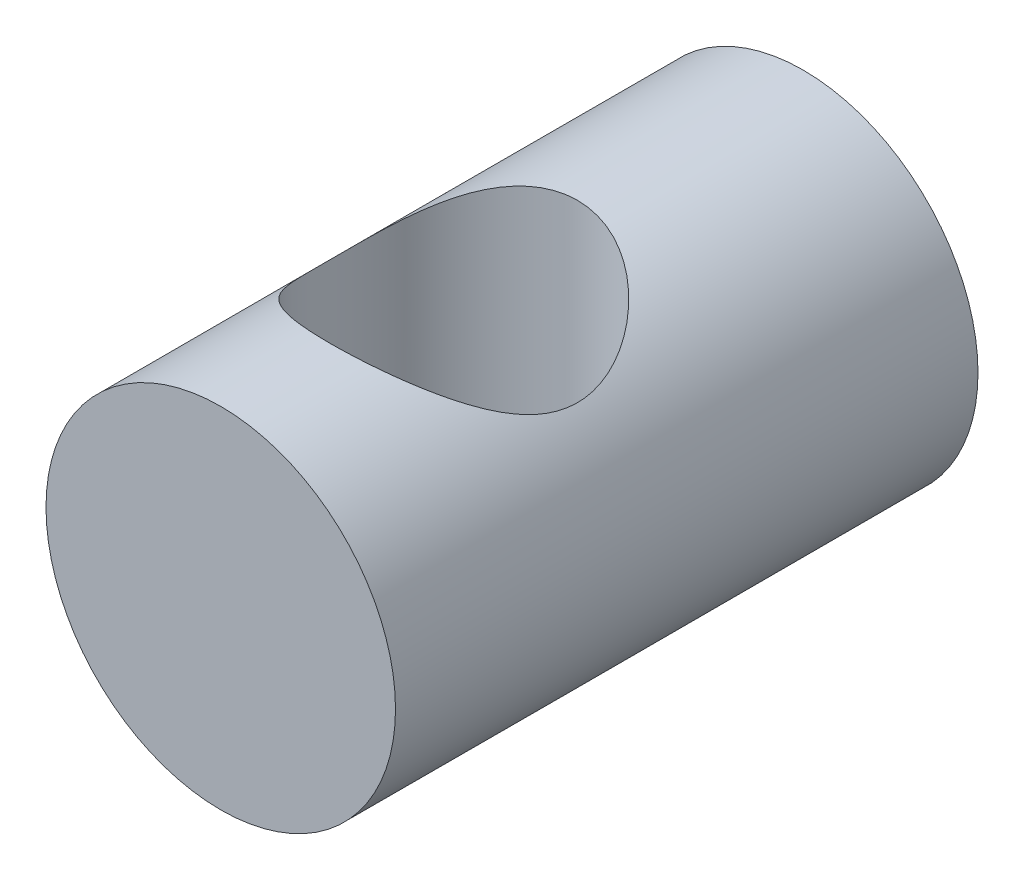
from build123d import *

# Parameters (mm, degrees)
SKETCH1_R              = 6
BOSS_EXTRUDE1_DEPTH    = 20
SKETCH5_W              = 4.25
SKETCH5_H              = 6
M10_TAPPED_HOLE1_D     = 8.5
M10_TAPPED_HOLE1_DEPTH = 27.5
M10_TAPPED_HOLE1_TIP   = 2.553657631


with BuildPart() as part:
    # Sketch1 → Boss-Extrude1 (new body)
    with BuildSketch(Plane.XY):
        Circle(SKETCH1_R)
    extrude(amount=BOSS_EXTRUDE1_DEPTH)

    # Sketch5 → M10 Tapped Hole2 (revolve, cut)
    with BuildSketch(Plane(origin=(0, 0, 12), x_dir=(0, 0, -1), z_dir=(1, 0, 0))):
        with Locations((2.125, 3)):
            Rectangle(SKETCH5_W, SKETCH5_H)
    revolve(axis=Axis((0, -6.35, 12), (0, 1, 0)), mode=Mode.SUBTRACT)

    # M10 Tapped Hole1
    with Locations(Plane(origin=(0, 0, 0), x_dir=(1, 0, 0), z_dir=(0, 1, 0))):
        with Locations((0, -12)):
            Hole(M10_TAPPED_HOLE1_D / 2, depth=M10_TAPPED_HOLE1_DEPTH)
            with Locations((0, 0, -(M10_TAPPED_HOLE1_DEPTH + M10_TAPPED_HOLE1_TIP / 2))):  # 118° drill point
                Cone(0, M10_TAPPED_HOLE1_D / 2, M10_TAPPED_HOLE1_TIP, mode=Mode.SUBTRACT)


solid = part.part
